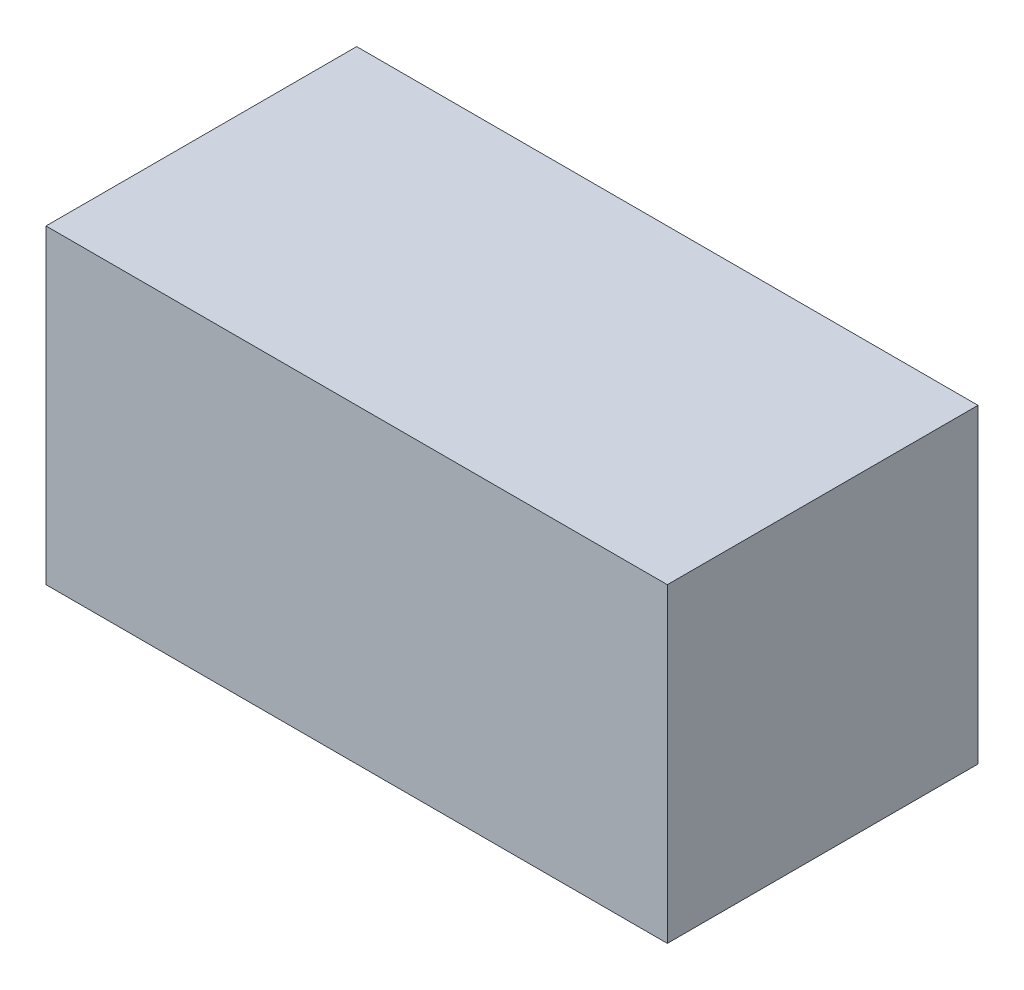
SolidWorks part; units mm, degrees
ref_plane "Front Plane" through (0, 0, 0) normal (0, 0, 1) x (1, 0, 0)
ref_plane "Top Plane" through (0, 0, 0) normal (0, 1, 0) x (1, 0, 0)
ref_plane "Right Plane" through (0, 0, 0) normal (1, 0, 0) x (0, 0, -1)
other "Configuration Table"
sketch "Sketch1" plane through (0, 0, 0) normal (0, 0, 1) x (1, 0, 0)
  line L1 (0, 0) -> (60, 0)
  line L2 (0, 0) -> (0, 30)
  line L3 (0, 30) -> (60, 30)
  line L4 (60, 0) -> (60, 30)
  dimension "D1" = 60
  dimension "D2" = 30
extrude "Boss-Extrude1" add sketch "Sketch1" along normal blind 30
